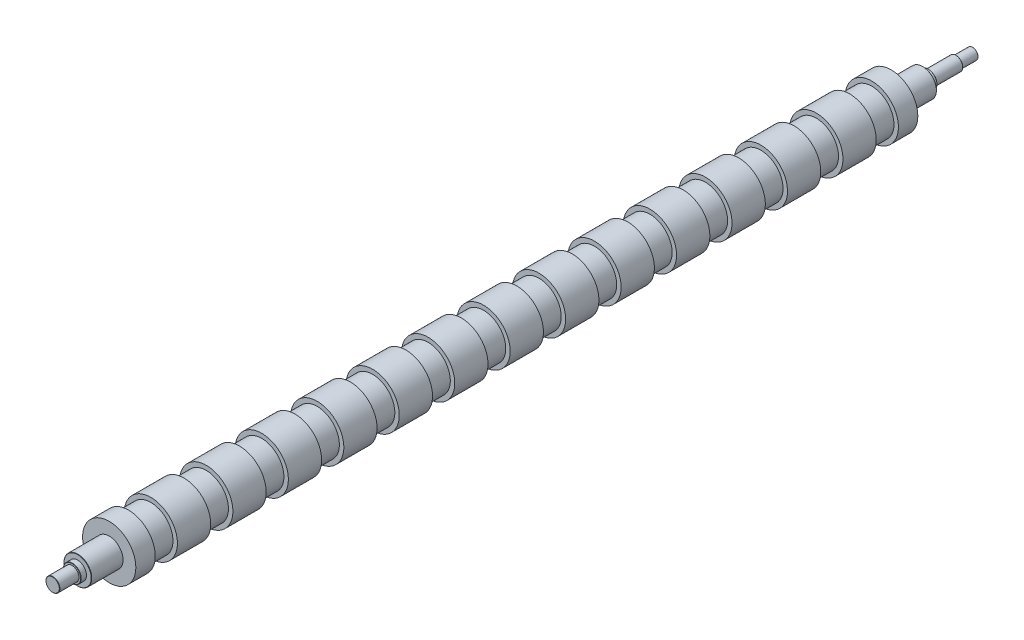
SolidWorks part; units mm, degrees
ref_plane "前视基准面" through (0, 0, 0) normal (0, 0, 1) x (1, 0, 0)
ref_plane "上视基准面" through (0, 0, 0) normal (0, 1, 0) x (1, 0, 0)
ref_plane "右视基准面" through (0, 0, 0) normal (1, 0, 0) x (0, 0, -1)
sketch "草图1" plane through (0, 0, 0) normal (0, 0, 1) x (1, 0, 0)
  circle A0 centre (0, 0) radius 48
  dimension "D1" = 96
extrude "凸台-拉伸1" add sketch "草图1" along normal blind 1410
sketch "草图2" plane through (0, 0, 1410) normal (0, 0, 1) x (1, 0, 0)
  circle A0 centre (0, 0) radius 16
  dimension "D1" = 32
extrude "凸台-拉伸2" add sketch "草图2" along normal blind 67
sketch "草图3" plane through (0, 0, 0) normal (0, 0, -1) x (-1, 0, 0)
  circle A0 centre (0, 0) radius 16
  dimension "D1" = 32
extrude "凸台-拉伸3" add sketch "草图3" along normal blind 67
sketch "草图4" plane through (0, 0, -67) normal (0, 0, -1) x (-1, 0, 0)
  circle A0 centre (0, 0) radius 12.5
  circle A1 centre (0, 0) radius 16 construction
  dimension "D1" = 25
extrude "凸台-拉伸4" add sketch "草图4" along normal blind 80
sketch "草图5" plane through (0, 0, 1477) normal (0, 0, 1) x (1, 0, 0)
  circle A0 centre (0, 0) radius 12.5
  circle A1 centre (0, 0) radius 16 construction
  dimension "D1" = 25
extrude "凸台-拉伸5" add sketch "草图5" along normal blind 35
sketch "草图6" plane through (0, 0, -147) normal (0, 0, -1) x (-1, 0, 0)
  circle A0 centre (0, 0) radius 10
  dimension "D1" = 20
extrude "切除-拉伸1" cut sketch "草图6" against normal blind 30 flip side to cut
sketch "草图7" plane through (0, 0, 0) normal (1, 0, 0) x (0, 0, -1)
  line L0 (-1410, -48) -> (0, -48) construction
  line L1 (-75, -48) -> (-35, -48)
  line L2 (-75, -48) -> (-75, -40)
  line L3 (-75, -40) -> (-35, -40)
  line L4 (-35, -48) -> (-35, -40)
  line L5 (0, -48) -> (0, 48) construction
  line L6 (0, 0) -> (-295.6624, 0) construction
  dimension "D1" = 35
  dimension "D2" = 40
  dimension "D3" = 8
revolve "切除-旋转1" cut sketch "草图7" angle 360 about L6
sketch "草图8" plane through (0, 0, 0) normal (0, 1, 0) x (1, 0, 0)
  line L0 (0, 181.2733) -> (0, 0)
pattern_linear "阵列(线性)1" count 14 spacing 100 along (0, 0, 1) of "切除-旋转1"
sketch "草图9" plane through (0, 0, 1410) normal (0, 0, 1) x (1, 0, 0)
  circle A0 centre (0, 0) radius 25
  dimension "D1" = 50
extrude "凸台-拉伸6" add sketch "草图9" along normal blind 57
sketch "草图10" plane through (0, 0, 0) normal (0, 0, -1) x (-1, 0, 0)
  circle A0 centre (0, 0) radius 25
  dimension "D1" = 50
extrude "凸台-拉伸7" add sketch "草图10" along normal blind 57
chamfer "倒角1" distance 0.5 angle 45 7 edges at (12.5, 0, 1512) (16, 0, 1477) (25, 0, 1467) (-25, 0, -57) (-16, 0, -67) (-12.5, 0, -117) (-10, 0, -147)
